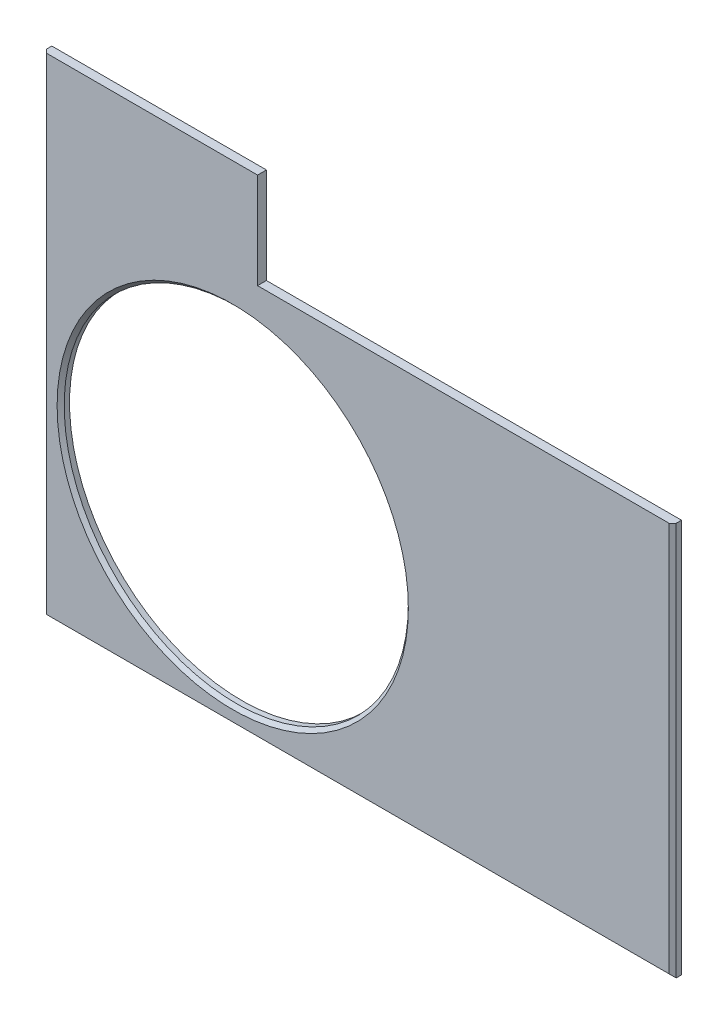
from build123d import *

# Parameters (mm, degrees)
SKETCH1_R           = 485
BOSS_EXTRUDE1_DEPTH = 25
CHAMFER1_SIZE       = 10


with BuildPart() as part:
    # Sketch1 → Boss-Extrude1 (new body)
    with BuildSketch(Plane.XY):
        Polygon((0, 0), (1775, 0), (1775, 1110), (605, 1110), (605, 1380), (0, 1380), align=None)
        with Locations((535, 535)):
            Circle(SKETCH1_R, mode=Mode.SUBTRACT)
    extrude(amount=BOSS_EXTRUDE1_DEPTH)

    # Chamfer1
    chamfer1_edges = [part.edges().sort_by_distance(p)[0] for p in [
        (1775, 555, 25),
        (50, 535, 25),
        (0, 690, 25),
        (887.5, 0, 25),
    ]]
    chamfer(chamfer1_edges, length=CHAMFER1_SIZE)


solid = part.part
